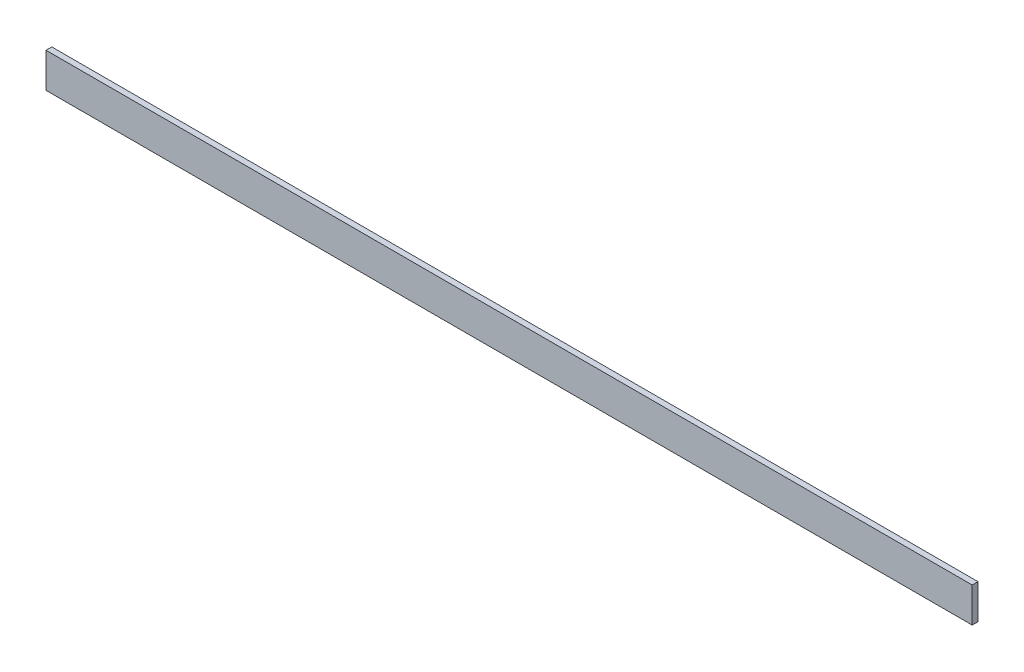
SolidWorks part; units mm, degrees
material "1023 碳钢板 (SS)"
ref_plane "Front Plane" through (0, 0, 0) normal (0, 0, 1) x (1, 0, 0)
ref_plane "Top Plane" through (0, 0, 0) normal (0, 1, 0) x (1, 0, 0)
ref_plane "Right Plane" through (0, 0, 0) normal (1, 0, 0) x (0, 0, -1)
sketch "Sketch1" plane through (0, 0, 0) normal (0, 0, 1) x (1, 0, 0)
  line L1 (-400, 15) -> (400, 15)
  line L2 (-400, 15) -> (-400, -15)
  line L3 (-400, -15) -> (400, -15)
  line L4 (400, 15) -> (400, -15)
  line L5 (-400, 15) -> (400, -15) construction
  line L6 (-400, -15) -> (400, 15) construction
  point P0 (0, 0)
  dimension "D1" = 800
  dimension "D2" = 30
extrude "Boss-Extrude1" add sketch "Sketch1" along normal blind 5
